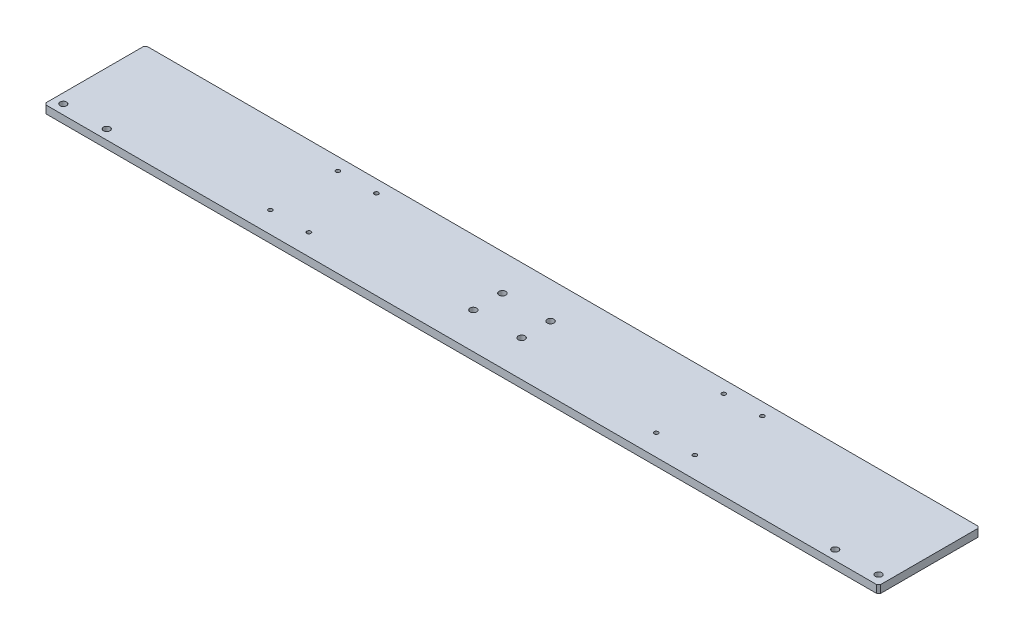
from build123d import *

# Parameters (mm, degrees)
SKETCH_1_W            = 865
SKETCH_1_H            = 105
EXTRUDE_1_DEPTH       = 4
CHAMFER_1_SIZE        = 2
HOLE_WIZARD_M5_1_D    = 4.2
HOLE_WIZARD_7_0_7_1_D = 7
HOLE_WIZARD_M8_1_D    = 6.8


with BuildPart() as part:
    # 草图1 → 凸台-拉伸1 (new, symmetric)
    with BuildSketch(Plane(origin=(0, 0, 0), x_dir=(1, 0, 0), z_dir=(0, 1, 0))):
        Rectangle(SKETCH_1_W, SKETCH_1_H)
    extrude(amount=EXTRUDE_1_DEPTH, both=True)

    # 倒角1
    chamfer_1_edges = [part.edges().sort_by_distance(p)[0] for p in [
        (432.5, 0, 52.5),
        (-432.5, 0, 52.5),
        (-432.5, 0, -52.5),
        (432.5, 0, -52.5),
    ]]
    chamfer(chamfer_1_edges, length=CHAMFER_1_SIZE)

    # M5 螺纹孔1 (through all)
    with Locations(Plane(origin=(0, 4, 0), x_dir=(1, 0, 0), z_dir=(0, 1, 0))):
        with Locations((-220, 39.5), (-180, 39.5), (-180, -30.5), (-220, -30.5), (220, -30.5), (180, -30.5), (180, 39.5), (220, 39.5)):
            Hole(HOLE_WIZARD_M5_1_D / 2)

    # Ø7.0 (7) 直径孔1 (through all)
    with Locations(Plane(origin=(0, 4, 0), x_dir=(1, 0, 0), z_dir=(0, 1, 0))):
        with Locations((25, -15), (25, 15), (-25, 15), (-25, -15)):
            Hole(HOLE_WIZARD_7_0_7_1_D / 2)

    # M8 螺纹孔1 (through all)
    with Locations(Plane(origin=(0, 4, 0), x_dir=(1, 0, 0), z_dir=(0, 1, 0))):
        with Locations((422.5, -42.5), (377.5, -42.5), (-377.5, -42.5), (-422.5, -42.5)):
            Hole(HOLE_WIZARD_M8_1_D / 2)


solid = part.part
